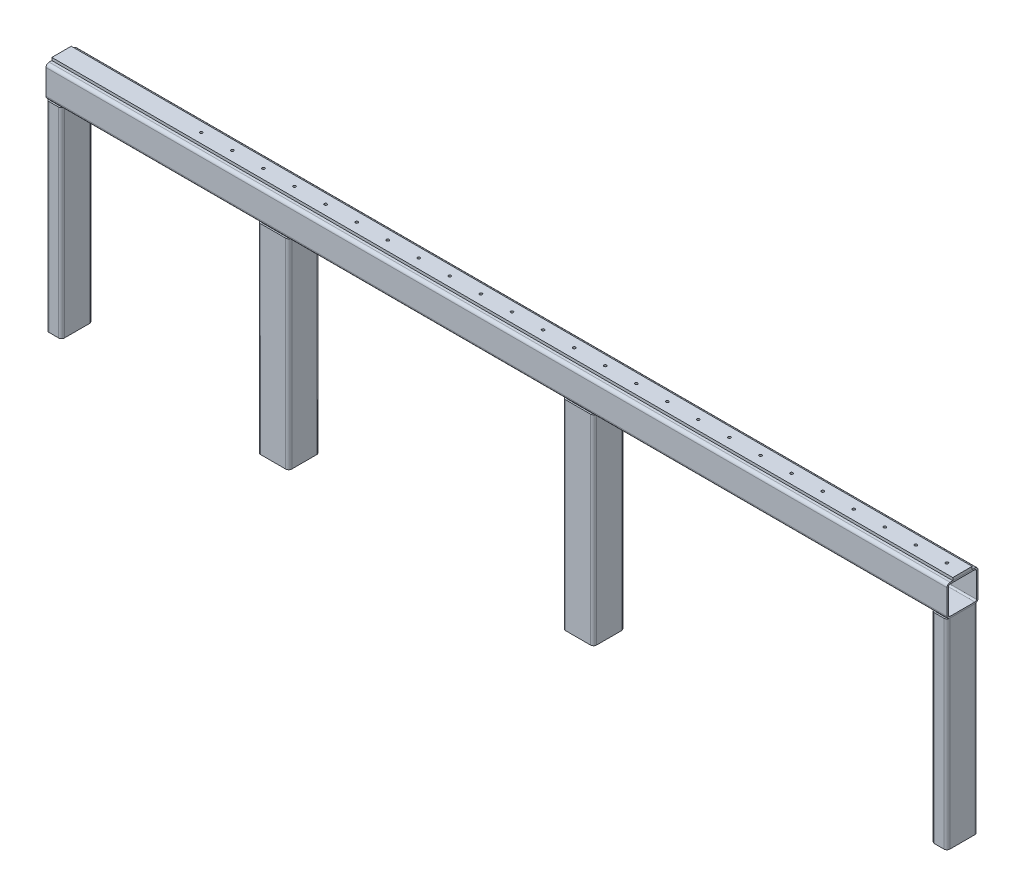
from build123d import *

# Parameters (mm, degrees)
GB_6728_1986_RECTANGULAR_HOLLOW_SECTION_DEPTH  = 515
GB_6728_1986_RECTANGULAR_HOLLOW_SECT_2_DEPTH   = 515
GB_6728_1986_SQUARE_HOLLOW_SECTION_080_X_DEPTH = 2280
BODY_START                                     = 226.27416998
BODY_3_RUN_ON_DEPTH                            = 246.27416998
BODY_START_2                                   = 2053.72583002
BODY_3_RUN_ON_2_DEPTH                          = 246.27416998
SKETCH2_W                                      = 2320
SKETCH2_H                                      = 50
BOSS_EXTRUDE1_DEPTH                            = 10
SKETCH4_W                                      = 2320
SKETCH4_H                                      = 50
CUT_EXTRUDE1_DEPTH                             = 3
LPATTERN1_COUNT                                = 25
LPATTERN1_PITCH                                = 80
SQUARE_TUBE_80_X_80_X_4_0_1_DEPTH              = 515
SQUARE_TUBE_80_X_80_X_4_0_1_2_DEPTH            = 515


with BuildPart() as part:
    # Sketch11 → Gb／6728-1986 Rectangular Hollow Section 080 X 40 X 4(1) (new body)
    with BuildSketch(Plane(origin=(0, 0, 0), x_dir=(-1, 0, 0), z_dir=(0, 1, 0))):
        with BuildLine():
            Line((-12, -40), (12, -40))
            ThreePointArc((12, -40), (17.656854249, -37.656854249), (20, -32))
            Line((20, -32), (20, 32))
            ThreePointArc((20, 32), (17.656854249, 37.656854249), (12, 40))
            Line((12, 40), (-12, 40))
            ThreePointArc((-12, 40), (-17.656854249, 37.656854249), (-20, 32))
            Line((-20, 32), (-20, -32))
            ThreePointArc((-20, -32), (-17.656854249, -37.656854249), (-12, -40))
        make_face()
        with BuildLine():
            Line((-12, -36), (12, -36))
            ThreePointArc((12, -36), (14.828427125, -34.828427125), (16, -32))
            Line((16, -32), (16, 32))
            ThreePointArc((16, 32), (14.828427125, 34.828427125), (12, 36))
            Line((12, 36), (-12, 36))
            ThreePointArc((-12, 36), (-14.828427125, 34.828427125), (-16, 32))
            Line((-16, 32), (-16, -32))
            ThreePointArc((-16, -32), (-14.828427125, -34.828427125), (-12, -36))
        make_face(mode=Mode.SUBTRACT)
    extrude(amount=GB_6728_1986_RECTANGULAR_HOLLOW_SECTION_DEPTH)


with BuildPart() as body_2:
    # Sketch11 on segment 2 (carried to segment 2) → Gb_6728-1986 Rectangular Hollow Sect 2 (new body)
    with BuildSketch(Plane(origin=(2280, 0, 0), x_dir=(-1, 0, 0), z_dir=(0, 1, 0))):
        with BuildLine():
            Line((-12, -40), (12, -40))
            ThreePointArc((12, -40), (17.656854249, -37.656854249), (20, -32))
            Line((20, -32), (20, 32))
            ThreePointArc((20, 32), (17.656854249, 37.656854249), (12, 40))
            Line((12, 40), (-12, 40))
            ThreePointArc((-12, 40), (-17.656854249, 37.656854249), (-20, 32))
            Line((-20, 32), (-20, -32))
            ThreePointArc((-20, -32), (-17.656854249, -37.656854249), (-12, -40))
        make_face()
        with BuildLine():
            Line((-12, -36), (12, -36))
            ThreePointArc((12, -36), (14.828427125, -34.828427125), (16, -32))
            Line((16, -32), (16, 32))
            ThreePointArc((16, 32), (14.828427125, 34.828427125), (12, 36))
            Line((12, 36), (-12, 36))
            ThreePointArc((-12, 36), (-14.828427125, 34.828427125), (-16, 32))
            Line((-16, 32), (-16, -32))
            ThreePointArc((-16, -32), (-14.828427125, -34.828427125), (-12, -36))
        make_face(mode=Mode.SUBTRACT)
    extrude(amount=GB_6728_1986_RECTANGULAR_HOLLOW_SECT_2_DEPTH)


with BuildPart() as body_3:
    # Sketch1 → Gb／6728-1986 Square Hollow Section 080 X 80 X 4(1) (new body)
    with BuildSketch(Plane(origin=(0, 555, 0), x_dir=(0, 1, 0), z_dir=(1, 0, 0))):
        with BuildLine():
            Line((-32, -40), (32, -40))
            ThreePointArc((32, -40), (37.656854249, -37.656854249), (40, -32))
            Line((40, -32), (40, 32))
            ThreePointArc((40, 32), (37.656854249, 37.656854249), (32, 40))
            Line((32, 40), (-32, 40))
            ThreePointArc((-32, 40), (-37.656854249, 37.656854249), (-40, 32))
            Line((-40, 32), (-40, -32))
            ThreePointArc((-40, -32), (-37.656854249, -37.656854249), (-32, -40))
        make_face()
        with BuildLine():
            Line((-32, -36), (32, -36))
            ThreePointArc((32, -36), (34.828427125, -34.828427125), (36, -32))
            Line((36, -32), (36, 32))
            ThreePointArc((36, 32), (34.828427125, 34.828427125), (32, 36))
            Line((32, 36), (-32, 36))
            ThreePointArc((-32, 36), (-34.828427125, 34.828427125), (-36, 32))
            Line((-36, 32), (-36, -32))
            ThreePointArc((-36, -32), (-34.828427125, -34.828427125), (-32, -36))
        make_face(mode=Mode.SUBTRACT)
    extrude(amount=GB_6728_1986_SQUARE_HOLLOW_SECTION_080_X_DEPTH)

    # body 3 cut square before the run-on
    split(bisect_by=Plane(origin=(226.27416998, 555, 0), x_dir=(0, 1, 0), z_dir=(1, 0, 0)), keep=Keep.TOP)

    # Sketch1 → body 3 run on (add)
    with BuildSketch(Plane(origin=(0, 555, 0), x_dir=(0, 1, 0), z_dir=(1, 0, 0)).offset(BODY_START)):
        with BuildLine():
            Line((-32, -40), (32, -40))
            ThreePointArc((32, -40), (37.656854249, -37.656854249), (40, -32))
            Line((40, -32), (40, 32))
            ThreePointArc((40, 32), (37.656854249, 37.656854249), (32, 40))
            Line((32, 40), (-32, 40))
            ThreePointArc((-32, 40), (-37.656854249, 37.656854249), (-40, 32))
            Line((-40, 32), (-40, -32))
            ThreePointArc((-40, -32), (-37.656854249, -37.656854249), (-32, -40))
        make_face()
        with BuildLine():
            Line((-32, -36), (32, -36))
            ThreePointArc((32, -36), (34.828427125, -34.828427125), (36, -32))
            Line((36, -32), (36, 32))
            ThreePointArc((36, 32), (34.828427125, 34.828427125), (32, 36))
            Line((32, 36), (-32, 36))
            ThreePointArc((-32, 36), (-34.828427125, 34.828427125), (-36, 32))
            Line((-36, 32), (-36, -32))
            ThreePointArc((-36, -32), (-34.828427125, -34.828427125), (-32, -36))
        make_face(mode=Mode.SUBTRACT)
    extrude(amount=-BODY_3_RUN_ON_DEPTH)

    # body 3 cut square before the run-on
    split(bisect_by=Plane(origin=(2053.72583002, 555, 0), x_dir=(0, -1, 0), z_dir=(-1, 0, 0)), keep=Keep.TOP)

    # Sketch1 → body 3 run on 2 (add)
    with BuildSketch(Plane(origin=(0, 555, 0), x_dir=(0, 1, 0), z_dir=(1, 0, 0)).offset(BODY_START_2)):
        with BuildLine():
            Line((-32, -40), (32, -40))
            ThreePointArc((32, -40), (37.656854249, -37.656854249), (40, -32))
            Line((40, -32), (40, 32))
            ThreePointArc((40, 32), (37.656854249, 37.656854249), (32, 40))
            Line((32, 40), (-32, 40))
            ThreePointArc((-32, 40), (-37.656854249, 37.656854249), (-40, 32))
            Line((-40, 32), (-40, -32))
            ThreePointArc((-40, -32), (-37.656854249, -37.656854249), (-32, -40))
        make_face()
        with BuildLine():
            Line((-32, -36), (32, -36))
            ThreePointArc((32, -36), (34.828427125, -34.828427125), (36, -32))
            Line((36, -32), (36, 32))
            ThreePointArc((36, 32), (34.828427125, 34.828427125), (32, 36))
            Line((32, 36), (-32, 36))
            ThreePointArc((-32, 36), (-34.828427125, 34.828427125), (-36, 32))
            Line((-36, 32), (-36, -32))
            ThreePointArc((-36, -32), (-34.828427125, -34.828427125), (-32, -36))
        make_face(mode=Mode.SUBTRACT)
    extrude(amount=BODY_3_RUN_ON_2_DEPTH)


with BuildPart() as body_4:
    # Sketch2 → Boss-Extrude1 (new body)
    with BuildSketch(Plane(origin=(0, 595, 0), x_dir=(1, 0, 0), z_dir=(0, 1, 0))):
        with Locations((1140, 0)):
            Rectangle(SKETCH2_W, SKETCH2_H)
    extrude(amount=BOSS_EXTRUDE1_DEPTH)

    # Sketch4 → Cut-Extrude1 (cut)
    with BuildSketch(Plane(origin=(0, 605, 0), x_dir=(1, 0, 0), z_dir=(0, 1, 0))):
        with Locations((1140, 0)):
            Rectangle(SKETCH4_W, SKETCH4_H)
    extrude(amount=-CUT_EXTRUDE1_DEPTH, mode=Mode.SUBTRACT)


with BuildPart() as m8_tapped_hole1_tool:
    # Sketch6 → M8 Tapped Hole1 (revolve)
    with BuildSketch(Plane(origin=(2260, 602, 0), x_dir=(0, 0, 1), z_dir=(1, 0, 0))):
        Polygon((0, 0), (0, 21.792926105), (3.4, 19.75), (3.4, 0), align=None)
    m8_tapped_hole1 = revolve(axis=Axis((2260, 608.35, 0), (0, -1, 0)))


with BuildPart() as body_3_1:
    add(body_3.part)

    # M8 Tapped Hole1: cut by m8_tapped_hole1_tool
    add(m8_tapped_hole1_tool.part, mode=Mode.SUBTRACT)


with BuildPart() as body_4_1:
    add(body_4.part)

    # M8 Tapped Hole1: cut by m8_tapped_hole1_tool
    add(m8_tapped_hole1_tool.part, mode=Mode.SUBTRACT)


with BuildPart() as lpattern1_tool:
    # LPattern1: M8 Tapped Hole1 ×25
    with Locations(*[(-i * LPATTERN1_PITCH, 0, 0) for i in range(1, LPATTERN1_COUNT)]):
        add(m8_tapped_hole1)


with BuildPart() as body_3_2:
    add(body_3_1.part)

    # LPattern1: cut by lpattern1_tool
    add(lpattern1_tool.part, mode=Mode.SUBTRACT)


with BuildPart() as body_4_2:
    add(body_4_1.part)

    # LPattern1: cut by lpattern1_tool
    add(lpattern1_tool.part, mode=Mode.SUBTRACT)


with BuildPart() as body_5:
    # Sketch12 → Square Tube 80 X 80 X 4.0(1) (new body)
    with BuildSketch(Plane(origin=(565, 515, 0), x_dir=(1, 0, 0), z_dir=(0, -1, 0))):
        with BuildLine():
            Line((-32, -40), (32, -40))
            ThreePointArc((32, -40), (37.656854249, -37.656854249), (40, -32))
            Line((40, -32), (40, 32))
            ThreePointArc((40, 32), (37.656854249, 37.656854249), (32, 40))
            Line((32, 40), (-32, 40))
            ThreePointArc((-32, 40), (-37.656854249, 37.656854249), (-40, 32))
            Line((-40, 32), (-40, -32))
            ThreePointArc((-40, -32), (-37.656854249, -37.656854249), (-32, -40))
        make_face()
        with BuildLine():
            Line((-32, -36), (32, -36))
            ThreePointArc((32, -36), (34.828427125, -34.828427125), (36, -32))
            Line((36, -32), (36, 32))
            ThreePointArc((36, 32), (34.828427125, 34.828427125), (32, 36))
            Line((32, 36), (-32, 36))
            ThreePointArc((-32, 36), (-34.828427125, 34.828427125), (-36, 32))
            Line((-36, 32), (-36, -32))
            ThreePointArc((-36, -32), (-34.828427125, -34.828427125), (-32, -36))
        make_face(mode=Mode.SUBTRACT)
    extrude(amount=SQUARE_TUBE_80_X_80_X_4_0_1_DEPTH)


with BuildPart() as body_6:
    # Sketch12 on segment 2 (carried to segment 2) → Square Tube 80 X 80 X 4.0_1 2 (new body)
    with BuildSketch(Plane(origin=(1350, 515, 0), x_dir=(1, 0, 0), z_dir=(0, -1, 0))):
        with BuildLine():
            Line((-32, -40), (32, -40))
            ThreePointArc((32, -40), (37.656854249, -37.656854249), (40, -32))
            Line((40, -32), (40, 32))
            ThreePointArc((40, 32), (37.656854249, 37.656854249), (32, 40))
            Line((32, 40), (-32, 40))
            ThreePointArc((-32, 40), (-37.656854249, 37.656854249), (-40, 32))
            Line((-40, 32), (-40, -32))
            ThreePointArc((-40, -32), (-37.656854249, -37.656854249), (-32, -40))
        make_face()
        with BuildLine():
            Line((-32, -36), (32, -36))
            ThreePointArc((32, -36), (34.828427125, -34.828427125), (36, -32))
            Line((36, -32), (36, 32))
            ThreePointArc((36, 32), (34.828427125, 34.828427125), (32, 36))
            Line((32, 36), (-32, 36))
            ThreePointArc((-32, 36), (-34.828427125, 34.828427125), (-36, 32))
            Line((-36, 32), (-36, -32))
            ThreePointArc((-36, -32), (-34.828427125, -34.828427125), (-32, -36))
        make_face(mode=Mode.SUBTRACT)
    extrude(amount=SQUARE_TUBE_80_X_80_X_4_0_1_2_DEPTH)


solid = Compound([part.part, body_2.part, body_3_2.part, body_4_2.part, body_5.part, body_6.part])
